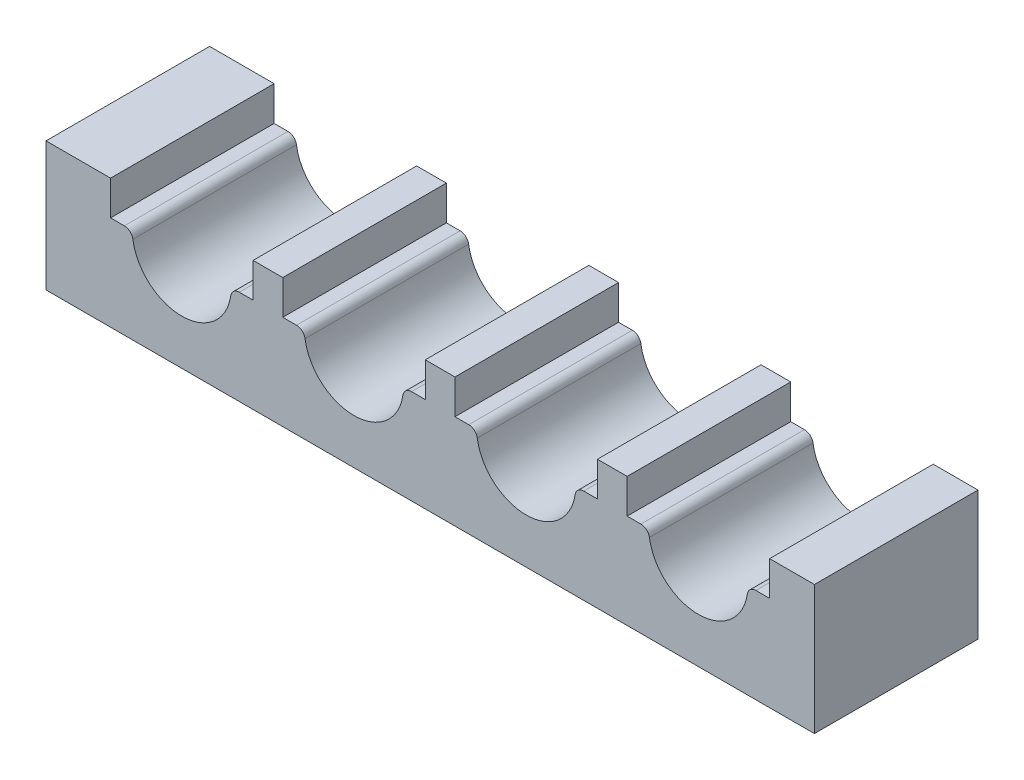
SolidWorks part; units mm, degrees
material "Q235A"
ref_plane "Front Plane" through (0, 0, 0) normal (0, 0, 1) x (1, 0, 0)
ref_plane "Top Plane" through (0, 0, 0) normal (0, 1, 0) x (1, 0, 0)
ref_plane "Right Plane" through (0, 0, 0) normal (1, 0, 0) x (0, 0, -1)
sketch "Sketch1" plane through (0, 0, 0) normal (0, 0, 1) x (1, 0, 0)
  line L1 (178.5, -30) -> (-178.5, -30)
  line L2 (178.5, -30) -> (178.5, 30)
  line L3 (178.5, 30) -> (-178.5, 30)
  line L4 (-178.5, -30) -> (-178.5, 30)
  line L5 (178.5, -30) -> (-178.5, 30) construction
  line L6 (178.5, 30) -> (-178.5, -30) construction
  point P0 (0, 0)
  dimension "D1" = 357
  dimension "D2" = 60
extrude "Boss-Extrude1" add sketch "Sketch1" along normal blind 76
sketch "Sketch2" plane through (0, 0, 76) normal (0, 0, 1) x (1, 0, 0)
  line L0 (178.5, 30) -> (-178.5, 30) construction
  line L1 (-82.3, 50) -> (-148.5, 50)
  line L2 (-82.3, 50) -> (-82.3, 14)
  line L3 (-82.3, 14) -> (-148.5, 14)
  line L4 (-148.5, 50) -> (-148.5, 14)
  line L5 (-82.3, 50) -> (-148.5, 14) construction
  line L6 (-82.3, 14) -> (-148.5, 50) construction
  line L7 (-178.5, 30) -> (-178.5, -30) construction
  point P0 (-115.4, 32)
  dimension "D1" = 66.2
  dimension "D2" = 16
  dimension "D3" = 30
extrude "Cut-Extrude1" cut sketch "Sketch2" against normal through all
sketch "Sketch3" plane through (0, 0, 76) normal (0, 0, 1) x (1, 0, 0)
  line L0 (-148.5, 14) -> (-82.3, 14) construction
  circle A0 centre (-115.4, 14) radius 23
  dimension "D1" = 46
extrude "Cut-Extrude2" cut sketch "Sketch3" against normal through all contours A0
fillet "Fillet1" radius 4 2 edges at (-138.4, 14, 38) (-92.4, 14, 38)
pattern_linear "LPattern1" count 4 spacing 80 along (1, 0, 0) of "Cut-Extrude1", "Cut-Extrude2", "Fillet1"
ref_plane "Plane1" through (-75.4, 0, 0) normal (1, 0, 0) x (0, 0, -1)
